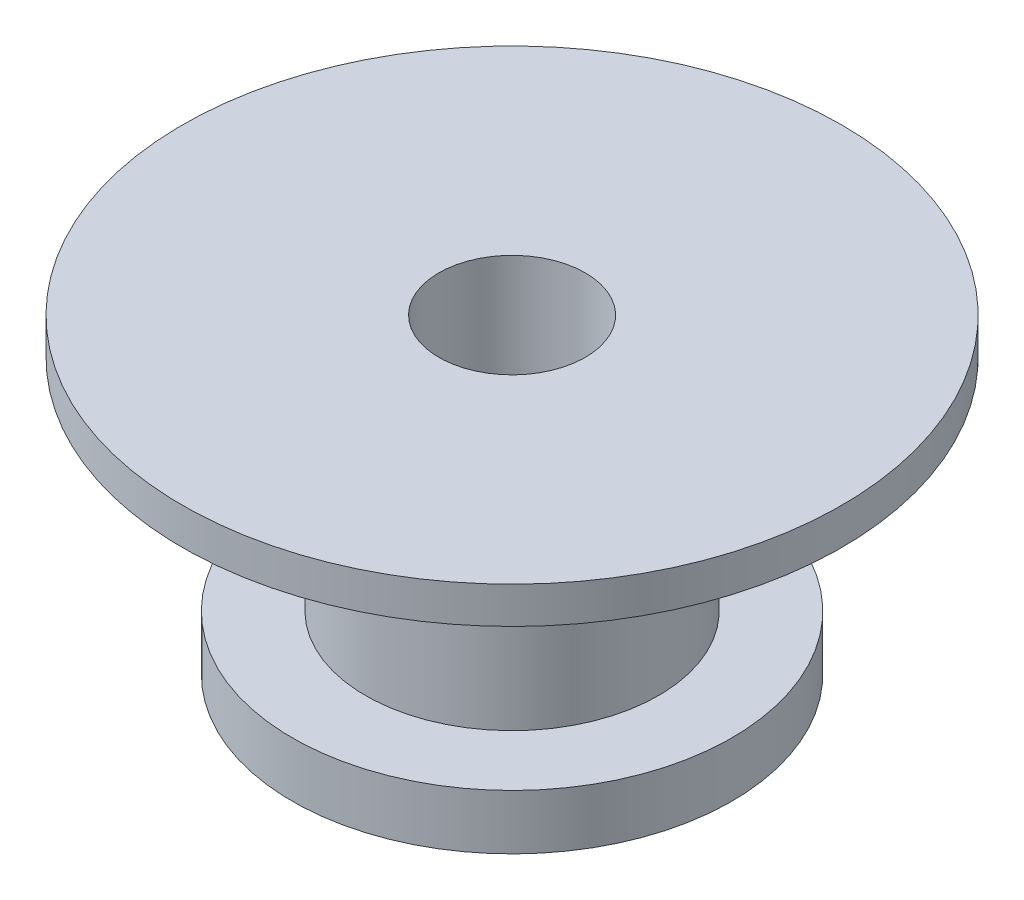
from build123d import *


with BuildPart() as part:
    # Sketch1 → Revolve1 (revolve)
    with BuildSketch(Plane.XY, mode=Mode.PRIVATE) as revolve1_sk:
        Polygon((2, 7), (2, -1.5), (6, -1.5), (6, 0), (4, 0), (4, 6), (9, 6), (9, 7), align=None)
    revolve(revolve1_sk.sketch.rotate(Axis((0, 0, 0), (0, 1, 0)), 90), axis=Axis((0, 0, 0), (0, 1, 0)))


solid = part.part
